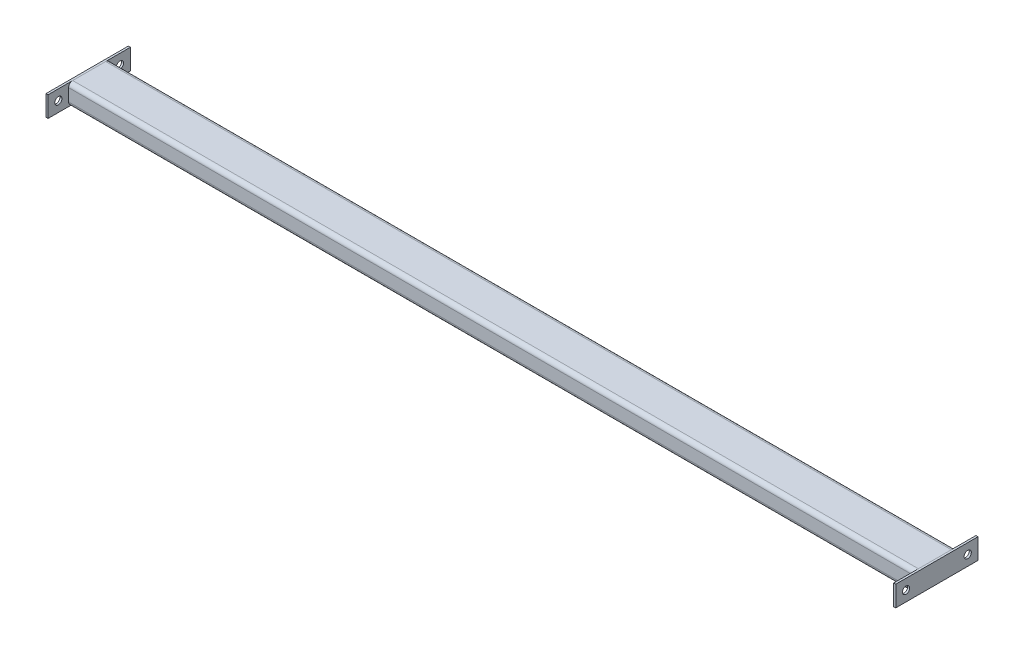
SolidWorks part; units mm, degrees
material "0Cr18Ni9Ti"
ref_plane "前视基准面" through (0, 0, 0) normal (0, 0, 1) x (1, 0, 0)
ref_plane "上视基准面" through (0, 0, 0) normal (0, 1, 0) x (1, 0, 0)
ref_plane "右视基准面" through (0, 0, 0) normal (1, 0, 0) x (0, 0, -1)
sketch "草图1" plane through (0, 0, 0) normal (0, 0, 1) x (1, 0, 0)
  line L0 (-617, 0) -> (617, 0)
  dimension "D1" = 1234
other "结构构件1"
ref_plane "基准面1" through (-617, 0, 0) normal (1, 0, 0) x (0, 1, 0)
sketch "Sketch1" plane through (-617, 0, 0) normal (1, 0, 0) x (0, 1, 0)
  line L0 (-9, -27) -> (9, -27)
  line L1 (-12, -24) -> (-12, 24)
  line L2 (9, 27) -> (-9, 27)
  line L3 (12, 24) -> (12, -24)
  line L4 (-9, -30) -> (9, -30)
  line L5 (-15, -24) -> (-15, 24)
  line L6 (9, 30) -> (-9, 30)
  line L7 (15, 24) -> (15, -24)
  arc A0 (15, 24) -> (9, 30) centre (9, 24) ccw
  arc A1 (9, -30) -> (15, -24) centre (9, -24) ccw
  arc A2 (-15, -24) -> (-9, -30) centre (-9, -24) ccw
  arc A3 (-9, 30) -> (-15, 24) centre (-9, 24) ccw
  arc A4 (-9, 27) -> (-12, 24) centre (-9, 24) ccw
  arc A5 (12, 24) -> (9, 27) centre (9, 24) ccw
  arc A6 (9, -27) -> (12, -24) centre (9, -24) ccw
  arc A7 (-12, -24) -> (-9, -27) centre (-9, -24) ccw
  point P0 (0, 30)
  point P1 (15, 0)
  point P2 (0, -30)
  point P3 (-15, 0)
  point P4 (-15, 30)
  point P5 (15, 30)
  point P6 (15, -30)
  point P7 (-15, -30)
  point P8 (0, 0)
  point P33 (0, 0)
sketch "草图3" plane through (617, 0, 0) normal (1, 0, 0) x (0, 0, -1)
  line L0 (24, 15) -> (-24, 15) construction
  line L1 (-60, -15) -> (60, -15)
  line L2 (-60, -15) -> (-60, 15)
  line L3 (-60, 15) -> (60, 15)
  line L4 (60, -15) -> (60, 15)
  line L5 (-60, -15) -> (60, 15) construction
  line L6 (-60, 15) -> (60, -15) construction
  line L7 (0, 0) -> (45, 0) construction
  line L8 (0, 0) -> (0, 15) construction
  circle A0 centre (45, 0) radius 5.25
  circle A1 centre (-45, 0) radius 5.25
  point P0 (0, 0)
  dimension "D2" = 10.5
  dimension "D3" = 45
  dimension "D1" = 120
extrude "凸台-拉伸1" add sketch "草图3" along normal blind 3 separate body
mirror "镜向1" about plane through (0, 0, 0) normal (1, 0, 0) of bodies 107
equation "\"D1@Sketch1\" = \"Thickness@Sketch1\" * 2"
